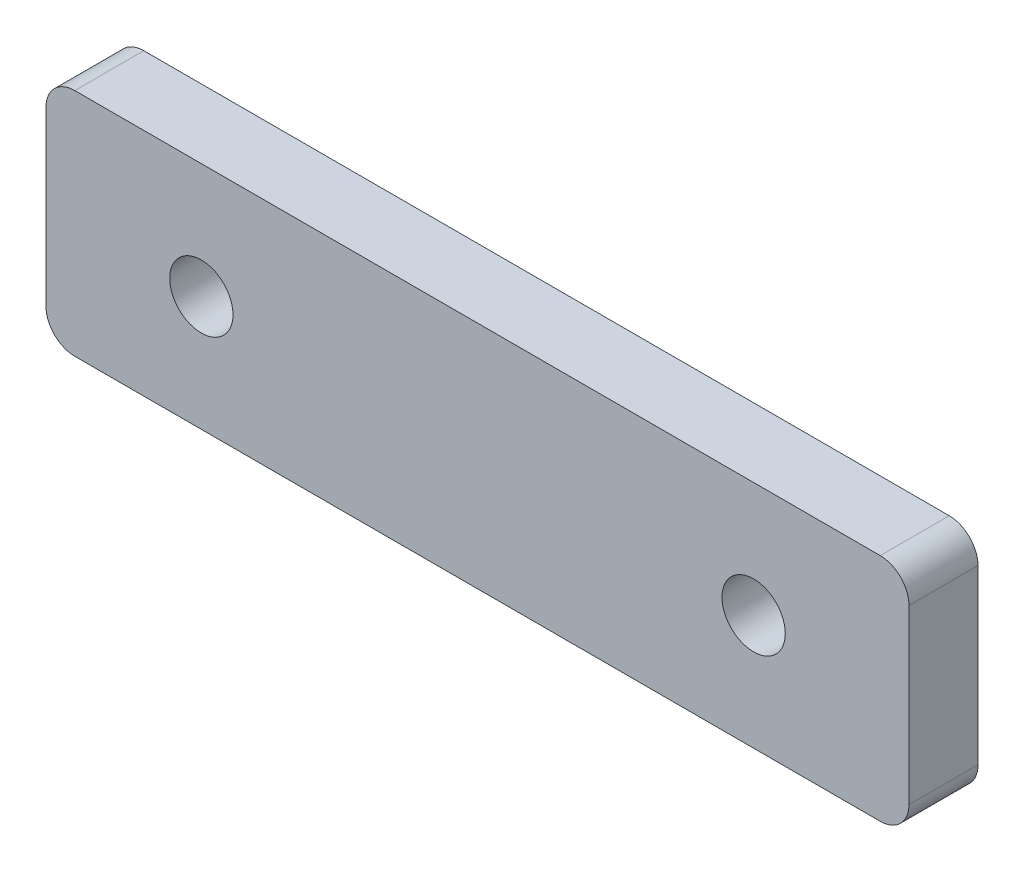
SolidWorks part; units mm, degrees
ref_plane "Front Plane" through (0, 0, 0) normal (0, 0, 1) x (1, 0, 0)
ref_plane "Top Plane" through (0, 0, 0) normal (0, 1, 0) x (1, 0, 0)
ref_plane "Right Plane" through (0, 0, 0) normal (1, 0, 0) x (0, 0, -1)
other "Configuration Table"
sketch "Sketch1" plane through (0, 0, 0) normal (0, 0, 1) x (1, 0, 0)
  line L1 (-75, -20) -> (75, -20)
  line L2 (-75, -20) -> (-75, 20)
  line L3 (-75, 20) -> (75, 20)
  line L4 (75, -20) -> (75, 20)
  line L5 (-75, -20) -> (75, 20) construction
  line L6 (-75, 20) -> (75, -20) construction
  point P0 (0, 0)
  dimension "D1" = 150
  dimension "D2" = 40
extrude "Boss-Extrude1" add sketch "Sketch1" along normal blind 12
sketch "Sketch2" plane through (0, 0, 12) normal (0, 0, 1) x (1, 0, 0)
  line L0 (-48, 0) -> (48, 0) construction
  line L1 (0, -20) -> (0, 20) construction
  line L2 (-75, -20) -> (75, -20) construction
  line L3 (75, 20) -> (-75, 20) construction
  circle A0 centre (-48, 0) radius 5.5
  circle A1 centre (48, 0) radius 5.5
  dimension "D3" = 11
  dimension "D4" = 11
  dimension "D1" = 96
  dimension "D2" = 48
extrude "Cut-Extrude1" cut sketch "Sketch2" against normal blind 8
fillet "Fillet1" radius 5 4 edges at (75, -20, 6) (75, 20, 6) (-75, -20, 6) (-75, 20, 6)
sketch "Sketch3" plane through (0, 0, 0) normal (0, 0, -1) x (-1, 0, 0)
  line L0 (-75, 0) -> (75, 0) construction
  line L1 (-75, -15) -> (-75, 15) construction
  line L2 (75, 15) -> (75, -15) construction
  circle A0 centre (-48, 0) radius 5.5
  circle A1 centre (48, 0) radius 5.5
  dimension "D3" = 11
  dimension "D4" = 11
  dimension "D1" = 96
  dimension "D2" = 48
extrude "Cut-Extrude2" cut sketch "Sketch3" against normal blind 12
